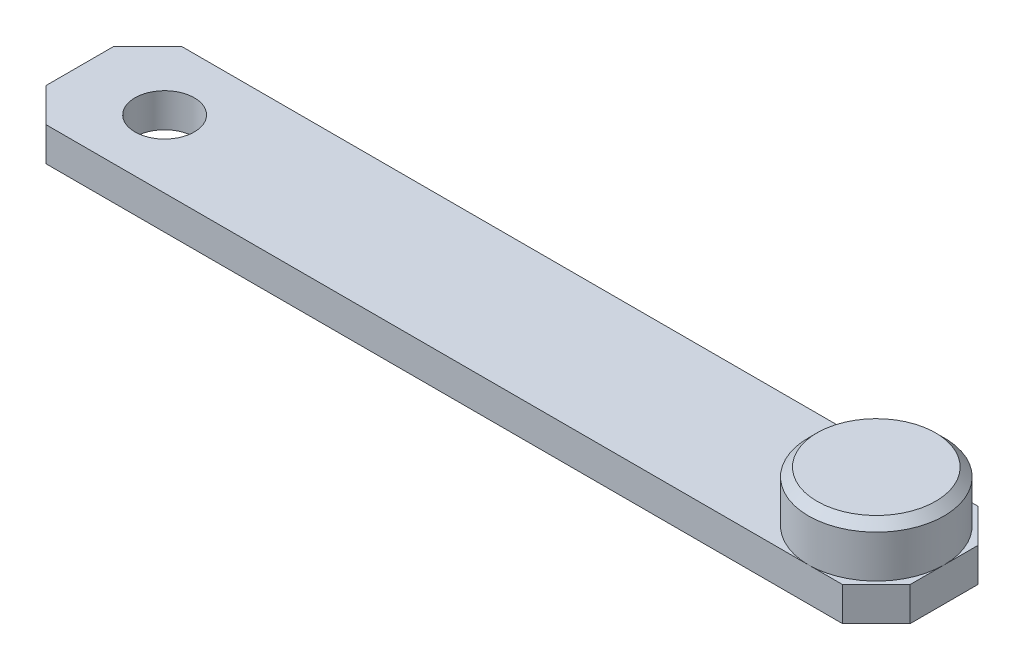
from build123d import *

# Parameters (mm, degrees)
SKETCH1_W           = 51
SKETCH1_H           = 8
BOSS_EXTRUDE1_DEPTH = 2
SKETCH2_R           = 1.75
CUT_EXTRUDE1_DEPTH  = 52.662365412
SKETCH3_R           = 4
BOSS_EXTRUDE2_DEPTH = 3
CHAMFER1_SIZE       = 0.5
CHAMFER2_SIZE       = 2


with BuildPart() as part:
    # Sketch1 → Boss-Extrude1 (new body)
    with BuildSketch(Plane(origin=(0, 0, 0), x_dir=(1, 0, 0), z_dir=(0, 1, 0))):
        with Locations((25.5, 4)):
            Rectangle(SKETCH1_W, SKETCH1_H)
    extrude(amount=BOSS_EXTRUDE1_DEPTH)

    # Sketch2 → Cut-Extrude1 (cut, through all)
    with BuildSketch(Plane(origin=(0, 2, 0), x_dir=(1, 0, 0), z_dir=(0, 1, 0))):
        with Locations(Location((5, 4, 0), (0, 0, 270))):
            Circle(SKETCH2_R)
    extrude(amount=-CUT_EXTRUDE1_DEPTH, mode=Mode.SUBTRACT)

    # Sketch3 → Boss-Extrude2 (add)
    with BuildSketch(Plane(origin=(0, 2, 0), x_dir=(1, 0, 0), z_dir=(0, 1, 0))):
        with Locations(Location((47, 4, 0), (0, 0, 270))):
            Circle(SKETCH3_R)
    extrude(amount=BOSS_EXTRUDE2_DEPTH)

    # Chamfer1
    chamfer1_edges = [part.edges().sort_by_distance(p)[0] for p in [
        (47, 5, -8),
    ]]
    chamfer(chamfer1_edges, length=CHAMFER1_SIZE)

    # Chamfer2
    chamfer2_edges = [part.edges().sort_by_distance(p)[0] for p in [
        (0, 1, -8),
        (51, 1, -8),
        (51, 1, 0),
        (0, 1, 0),
    ]]
    chamfer(chamfer2_edges, length=CHAMFER2_SIZE)


solid = part.part
